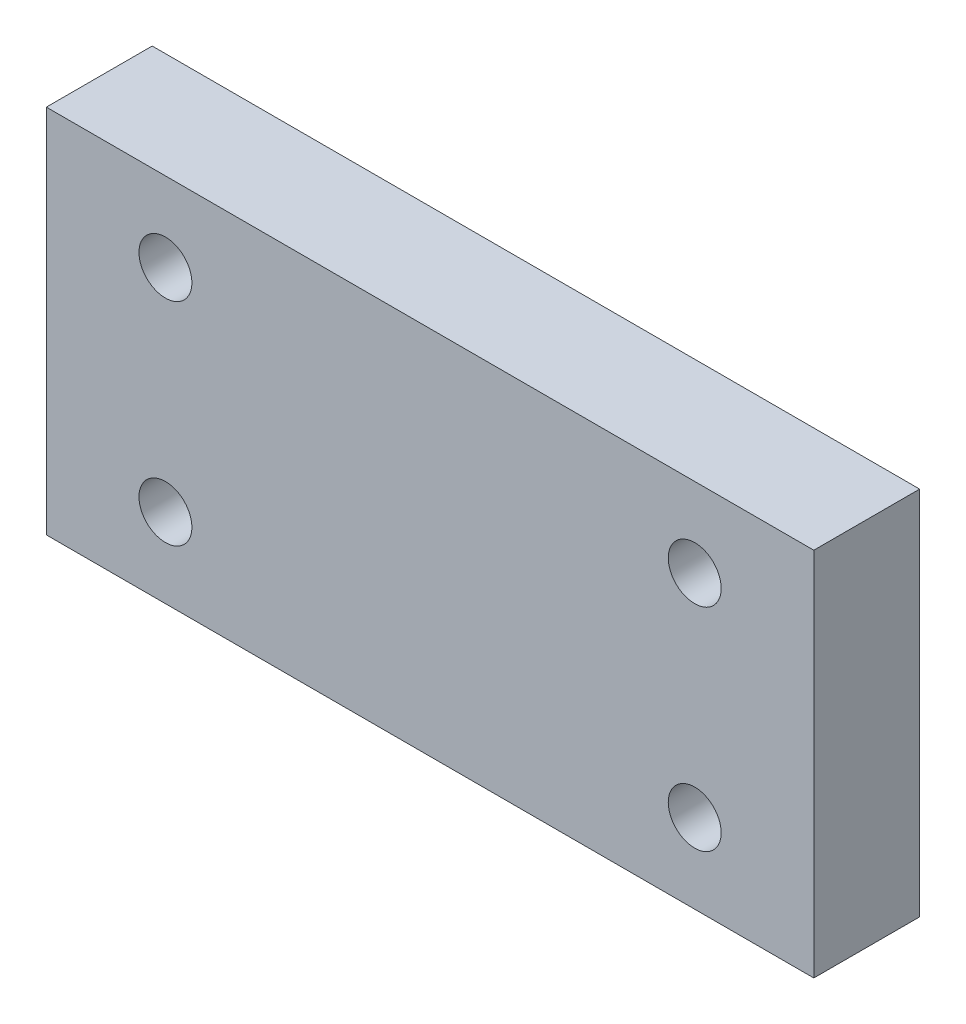
from build123d import *

# Parameters (mm, degrees)
SKETCH1_W           = 290
SKETCH1_H           = 140
SKETCH1_R           = 10
BOSS_EXTRUDE1_DEPTH = 40


with BuildPart() as part:
    # Sketch1 → Boss-Extrude1 (new body)
    with BuildSketch(Plane.XY):
        Rectangle(SKETCH1_W, SKETCH1_H)
        with Locations((-100, 40)):
            Circle(SKETCH1_R, mode=Mode.SUBTRACT)
        with Locations((100, 40)):
            Circle(SKETCH1_R, mode=Mode.SUBTRACT)
        with Locations(Location((100, -40, 0), (0, 0, 180))):
            Circle(SKETCH1_R, mode=Mode.SUBTRACT)
        with Locations(Location((-100, -40, 0), (0, 0, 180))):
            Circle(SKETCH1_R, mode=Mode.SUBTRACT)
    extrude(amount=BOSS_EXTRUDE1_DEPTH)


solid = part.part
